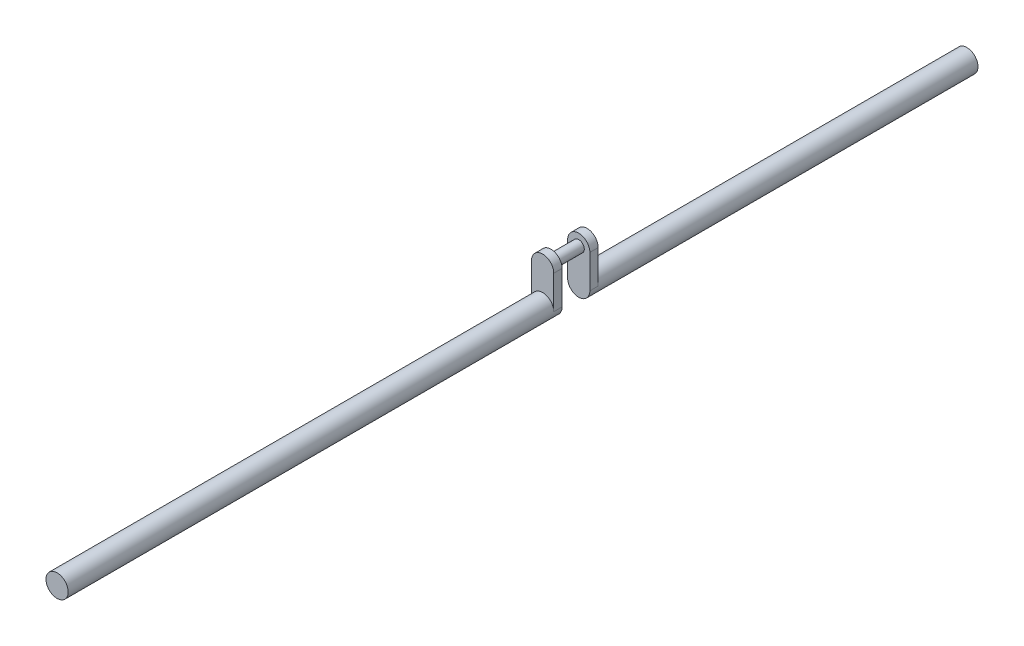
SolidWorks part; units mm, degrees
ref_plane "Front Plane" through (0, 0, 0) normal (0, 0, 1) x (1, 0, 0)
ref_plane "Top Plane" through (0, 0, 0) normal (0, 1, 0) x (1, 0, 0)
ref_plane "Right Plane" through (0, 0, 0) normal (1, 0, 0) x (0, 0, -1)
other "Configuration Table"
sketch "Sketch1" plane through (0, 0, 0) normal (0, 0, 1) x (1, 0, 0)
  circle A0 centre (0, 0) radius 10
  dimension "D1" = 20
extrude "Boss-Extrude1" add sketch "Sketch1" along normal mid plane 724
sketch "Sketch2" plane through (0, 0, 0) normal (0, 1, 0) x (1, 0, 0)
  line L1 (-72.5404, 20) -> (72.5404, 20)
  line L2 (-72.5404, 20) -> (-72.5404, -20)
  line L3 (-72.5404, -20) -> (72.5404, -20)
  line L4 (72.5404, 20) -> (72.5404, -20)
  line L5 (-72.5404, 20) -> (72.5404, -20) construction
  line L6 (-72.5404, -20) -> (72.5404, 20) construction
  point P0 (0, 0)
  dimension "D1" = 40
extrude "Cut-Extrude1" cut sketch "Sketch2" against normal through all both and the other way through all
sketch "Sketch3" plane through (0, 0, 0) normal (0, 0, 1) x (1, 0, 0)
  line L0 (0, 0) -> (0, 30) construction
  line L1 (-10, 0) -> (-10, 30)
  line L2 (10, 0) -> (10, 30)
  arc A0 (-10, 0) -> (10, 0) centre (0, 0) ccw
  arc A1 (10, 30) -> (-10, 30) centre (0, 30) ccw
  point P3 (0, 15)
  dimension "D1" = 10
  dimension "D2" = 30
extrude "Boss-Extrude2" add sketch "Sketch3" along normal mid plane 40
sketch "Sketch4" plane through (10, 0, 0) normal (1, 0, 0) x (0, 0, -1)
  line L1 (-12.5, 105.4811) -> (12.5, 105.4811)
  line L2 (-12.5, 105.4811) -> (-12.5, -105.4811)
  line L3 (-12.5, -105.4811) -> (12.5, -105.4811)
  line L4 (12.5, 105.4811) -> (12.5, -105.4811)
  line L5 (-12.5, 105.4811) -> (12.5, -105.4811) construction
  line L6 (-12.5, -105.4811) -> (12.5, 105.4811) construction
  point P0 (0, 0)
  dimension "D1" = 25
extrude "Cut-Extrude2" cut sketch "Sketch4" against normal through all both and the other way through all
sketch "Sketch5" plane through (0, 0, 0) normal (0, 0, 1) x (1, 0, 0)
  circle A0 centre (0, 30) radius 5
  dimension "D1" = 10
extrude "Boss-Extrude3" add sketch "Sketch5" along normal mid plane 25
sketch "Sketch6" plane through (0, 0, 362) normal (0, 0, 1) x (1, 0, 0)
  circle A1 centre (0, 0) radius 10
  circle A2 centre (0, 0) radius 10
  dimension "D1" = 0
extrude "Boss-Extrude4" add sketch "Sketch6" along normal blind 95.2
